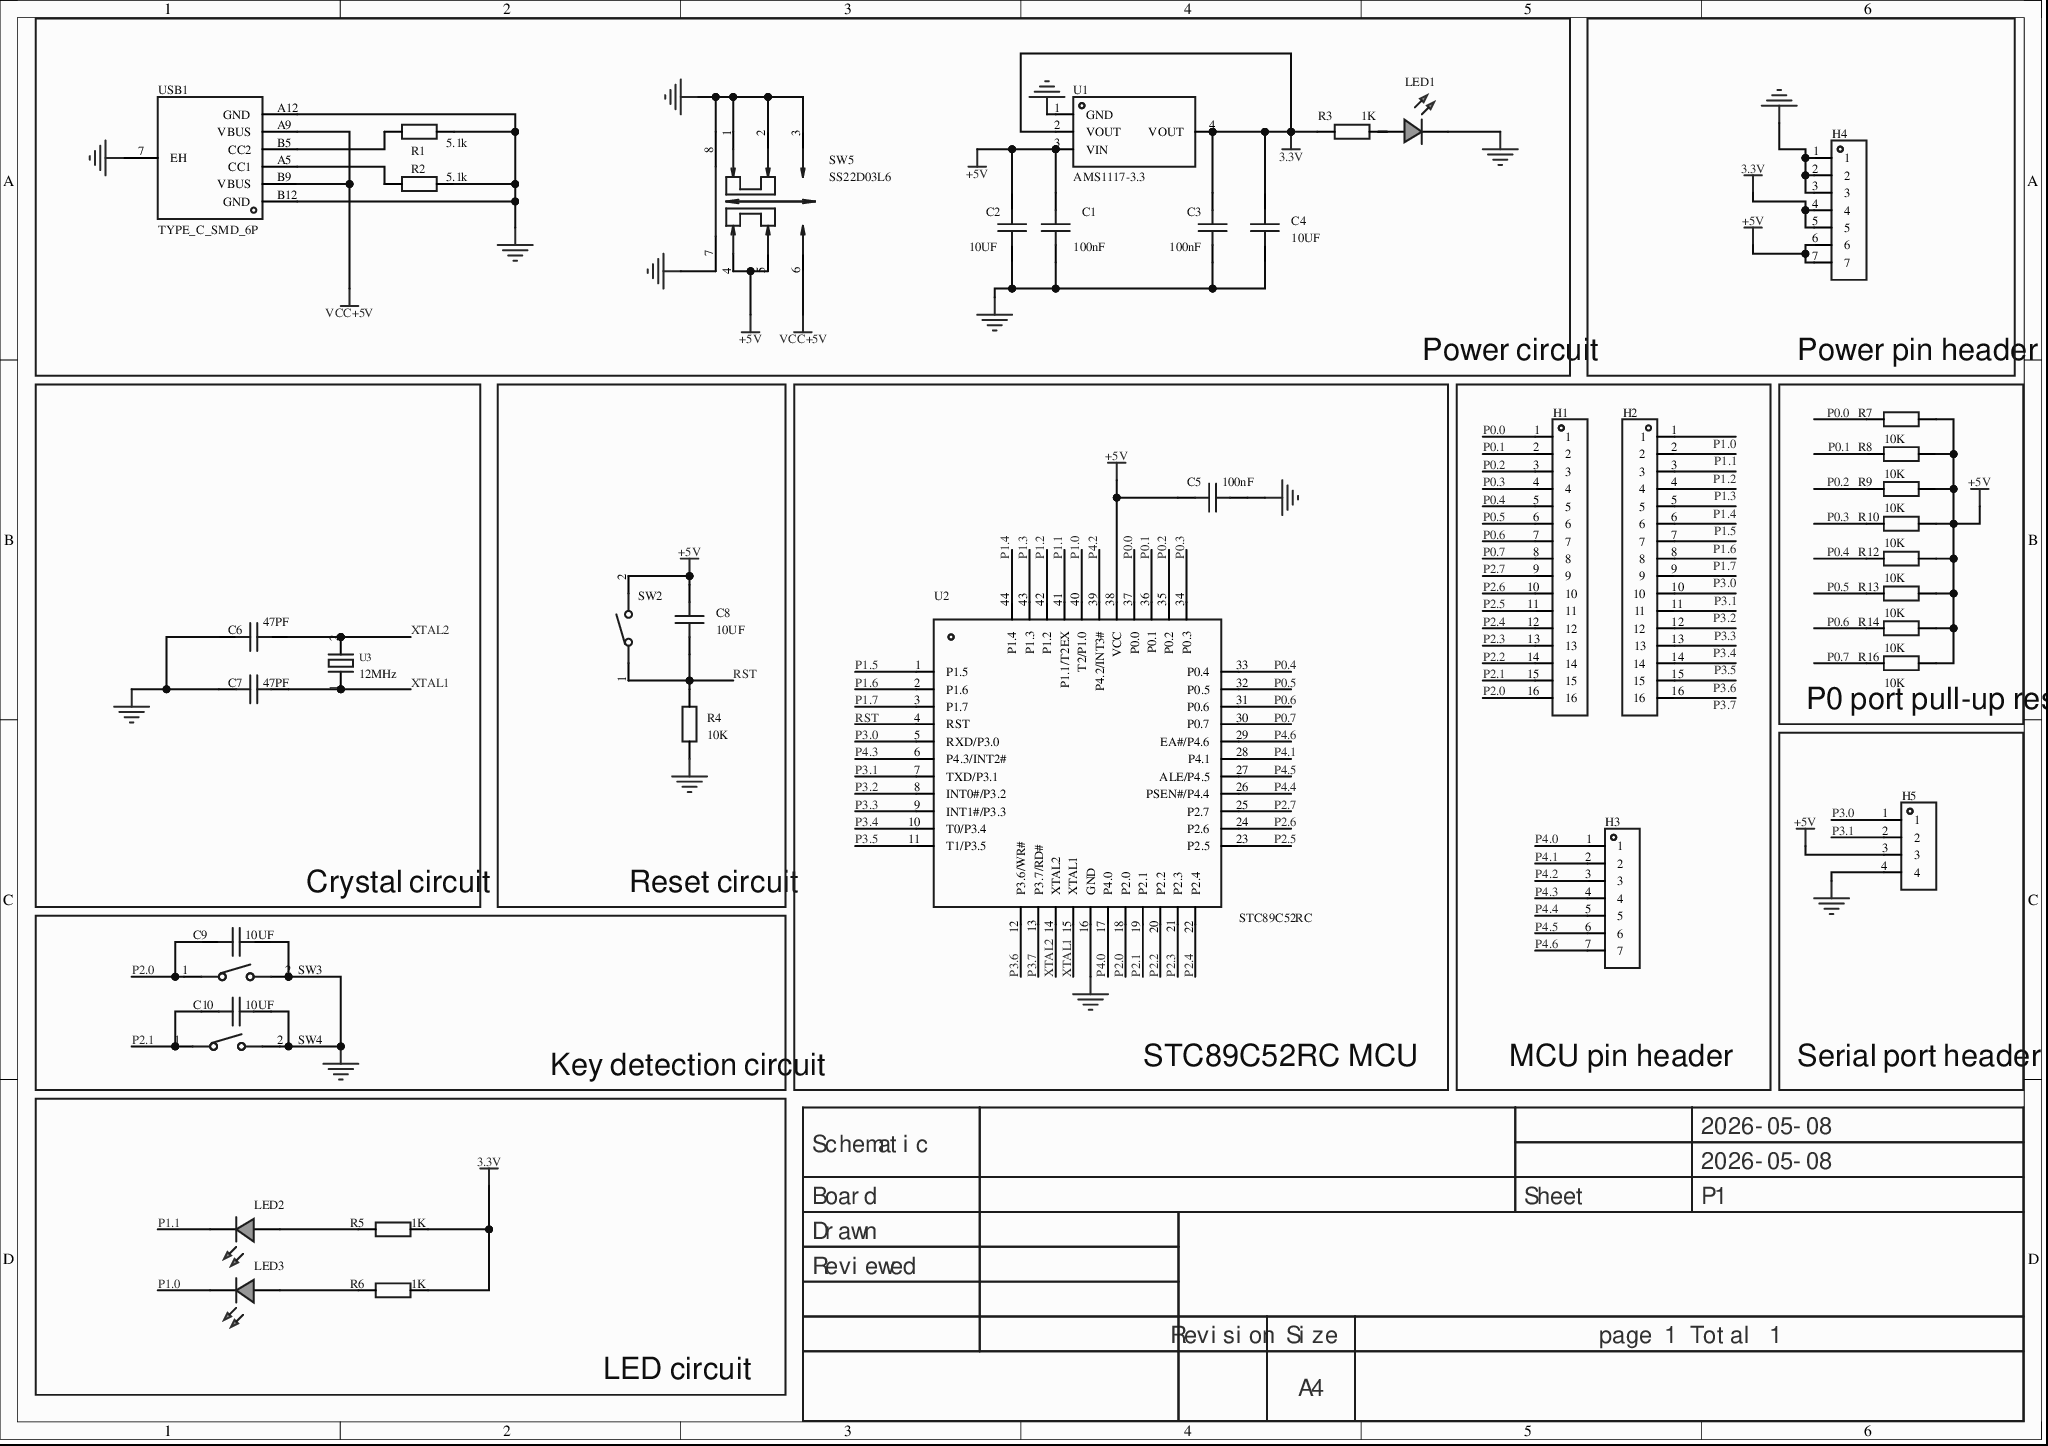
[diagram p0: MISC51716-3.schdoc]
# Altium project MISC51716-2.PrjPcb
1 sheet, 40 parts. Net scope: global (net labels, ports and power ports of the same name join across sheets).
Board file: MISC51716.pcbdoc

## Sheet MISC51716-3.schdoc
size 297 x 209 mm; Version: V1.0; @Project Name: MISC51716; @Update Date: 2026-05-08; @Create Date: 2026-05-08; @Board Name: MISC51716; @Create Time: 11:26:09; @Page Count: 1; @Page No: 1; @Schematic Name: MISC51716; @Update Time: 11:26:09; Size: A4

### Parts
C1  100nF  [C0805]
C2  10UF  [C0805]
C3  100nF  [C0805]
C4  10UF  [C0805]
C5  100nF  [C0805]
C6  47PF  [C0805]
C7  47PF  [C0805]
C8  10UF  [C0805]
C9  10UF  [C0805]
C10  10UF  [C0805]
H1  (no value)  [HDR-TH_16P-P2.54-V-M]
H2  (no value)  [HDR-TH_16P-P2.54-V-M]
H3  (no value)  [HDR-TH_7P-P2.54-V-M]
H4  (no value)  [HDR-TH_7P-P2.54-V-M]
H5  (no value)  [HDR-TH_4P-P2.54-V-M]
LED1  (no value)  [LED_0805]
LED2  (no value)  [LED_0805]
LED3  (no value)  [LED_0805]
R1  5.1k  [R0805]
R2  5.1k  [R0805]
R3  1K  [R0603]
R4  10K  [R0805]
R5  1K  [R0805]
R6  1K  [R0805]
R7  10K  [R0805]
R8  10K  [R0805]
R9  10K  [R0805]
R10  10K  [R0805]
R12  10K  [R0805]
R13  10K  [R0805]
R14  10K  [R0805]
R16  10K  [R0805]
SW2  Tact switch 3*4*H  [SW-SMD_L4.0-W2.9-LS5.0]  (value not drawn)
SW3  Tact switch 3*4*H  [SW-SMD_L4.0-W2.9-LS5.0]  (value not drawn)
SW4  Tact switch 3*4*H  [SW-SMD_L4.0-W2.9-LS5.0]  (value not drawn)
SW5  SS22D03L6  [SW-TH_SS-22D03-L4]
U1  AMS1117-3.3  [SOT-223-3_L6.5-W3.4-P2.30-LS7.0-BR]
U2  STC89C52RC  [LQFP-44_L10.0-W10.0-P0.80-LS12.0-BL]
U3  12MHz  [CRYSTAL-SMD_L11.4-W4.7-LS12.7]
USB1  TYPE_C_SMD_6P  [TYPE-C-SMD_TYPE-C-6P]

### Blocks framed on the sheet
Power circuit: C1-C4 LED1 R1-R3 SW5 U1 USB1
Power pin header: H4
Crystal circuit: C6 C7 U3
Reset circuit: C8 R4 SW2
MCU pin header: H1-H3

### Nets
3.3V: C3.2 C4.2 H4.4 H4.5 R3.1 R5.2 R6.2 U1.2(VOUT) U1.4(VOUT)
+5V: C1.2 C2.2 C5.2 C8.1 H4.6 H4.7 H5.3 R7.1 R8.1 R9.1 R10.1 R12.1 R13.1 R14.1 R16.1 SW2.2 SW5.4 SW5.5 U1.3(VIN) U2.38(VCC)
GND: C1.1 C2.1 C3.1 C4.1 C5.1 C6.2 C7.2 C9.1 C10.1 H4.1 H4.2 H4.3 H5.4 LED1.1(C) R1.2 R2.2 R4.1 SW3.2 SW4.2 SW5.1 SW5.2 SW5.3 SW5.7 SW5.8 U1.1(GND) U2.16(GND) USB1.7(EH) USB1.A12(GND) USB1.B12(GND)
VCC+5V: SW5.6 USB1.A9(VBUS) USB1.B9(VBUS)
P0.0: H1.1 R7.2 U2.37(P0.0)
P0.1: H1.2 R8.2 U2.36(P0.1)
P0.2: H1.3 R9.2 U2.35(P0.2)
P0.3: H1.4 R10.2 U2.34(P0.3)
P0.4: H1.5 R12.2 U2.33(P0.4)
P0.5: H1.6 R13.2 U2.32(P0.5)
P0.6: H1.7 R14.2 U2.31(P0.6)
P0.7: H1.8 R16.2 U2.30(P0.7)
P1.0: H2.1 LED3.1(C) U2.40(T2/P1.0)
P1.1: H2.2 LED2.1(C) U2.41(P1.1/T2EX)
P1.2: H2.3 U2.42(P1.2)
P1.3: H2.4 U2.43(P1.3)
P1.4: H2.5 U2.44(P1.4)
P1.5: H2.6 U2.1(P1.5)
P1.6: H2.7 U2.2(P1.6)
P1.7: H2.8 U2.3(P1.7)
P2.0: C9.2 H1.16 SW3.1 U2.18(P2.0)
P2.1: C10.2 H1.15 SW4.1 U2.19(P2.1)
P2.2: H1.14 U2.20(P2.2)
P2.3: H1.13 U2.21(P2.3)
P2.4: H1.12 U2.22(P2.4)
P2.5: H1.11 U2.23(P2.5)
P2.6: H1.10 U2.24(P2.6)
P2.7: H1.9 U2.25(P2.7)
P3.0: H2.9 H5.1 U2.5(RXD/P3.0)
P3.1: H2.10 H5.2 U2.7(TXD/P3.1)
P3.2: H2.11 U2.8(INT0#/P3.2)
P3.3: H2.12 U2.9(INT1#/P3.3)
P3.4: H2.13 U2.10(T0/P3.4)
P3.5: H2.14 U2.11(T1/P3.5)
P3.6: H2.15 U2.12(P3.6/WR#)
P3.7: H2.16 U2.13(P3.7/RD#)
P4.0: H3.1 U2.17(P4.0)
P4.1: H3.2 U2.28(P4.1)
P4.2: H3.3 U2.39(P4.2/INT3#)
P4.3: H3.4 U2.6(P4.3/INT2#)
P4.4: H3.5 U2.26(PSEN#/P4.4)
P4.5: H3.6 U2.27(ALE/P4.5)
P4.6: H3.7 U2.29(EA#/P4.6)
RST: C8.2 R4.2 SW2.1 U2.4(RST)
XTAL1: C7.1 U2.15(XTAL1) U3.1
XTAL2: C6.1 U2.14(XTAL2) U3.2(GND)
NetLED1_2: LED1.2(A) R3.2
NetLED2_2: LED2.2(A) R5.1
NetLED3_2: LED3.2(A) R6.1
NetR1_1: R1.1 USB1.B5(CC2)
NetR2_1: R2.1 USB1.A5(CC1)

### Notes on the sheet
- (near R16) P0 port pull-up resistors
- Key detection circuit
- STC89C52RC MCU
- Serial port header
- LED circuit
- 2026-05-08
- Schematic
- Board
- Sheet
- P1
- Drawn
- Reviewed
- Revision
- Size
- A4
- page 1 Total 1

### Library data of the parts
C1-C10 = CAP_0805: Symbol: CapAcitance; 3D Model: 1ba041120af144c991958decab20d241; 3D Model Transform: 78.74,51.181,0,0,0,0,0,0.0005,0; ConvertToPcb: yes; ModelName: C0805_L2.0-W1.3-H1.3; Device: CAP_0805; Supplier Footprint: 0805; AddInBom: yes; FootprintName: C0805
  C1 C3 C5: Value: 100nF
  C2 C4 C8-C10: Value: 10UF
  C6 C7: Value: 47PF
H1 H2 = HDR-M_2.54_1x16P: Pitch: 2.54mm; Total pins: 16; Rows: 1; Pin structure: 1x16P; Row spacing: -; Mounting type: Through-hole; Round/square pin: Square; Rated current: 3A; Rated voltage: -; Mating pin length: 6mm; Plastic height: 2.5mm; Termination pin length: 3mm; Contact material: -; Operating temp: -40℃~+105℃; Color: Black;; Symbol: HDR_2.54-1x16P; 3D Model: 8bf9bf52ab1b4a9c8444131cb972ade8; 3D Model Transform: 1590.1543,92.913,0,0,0,0,0,0,-137.795; ConvertToPcb: yes; ModelName: HDR-TH_16P-P2.54-M-LI-1X16P; Device: HDR-M_2.54_1x16P; Supplier Part: C2894939; Supplier Footprint: 插件; AddInBom: yes; FootprintName: HDR-TH_16P-P2.54-V-M
H3 H4 = HDR-M_2.54_1x7P: Symbol: PZ254V-11-07P; 3D Model: 3f496cdc752348c6a5e9157bbaceaf96; 3D Model Transform: 690.1561,98.425,0,0,0,0,0,0,-118.11; ConvertToPcb: yes; ModelName: HDR-TH_7P-P2.54-M-LI-1X7P; Device: HDR-M_2.54_1x7P; Supplier Part: C492406; Supplier Footprint: 插件; AddInBom: yes; FootprintName: HDR-TH_7P-P2.54-V-M
H5 = HDR-M_2.54_1x4P: Symbol: PZ254V-11-04P; 3D Model: 112f4d05e8d64e99ab9a333894bea4f9; 3D Model Transform: 399.999,104.7242,0,0,0,0,0,0,-118.11; ConvertToPcb: yes; ModelName: HDR-TH_4P-P2.54-M-LI-1X4P; Device: HDR-M_2.54_1x4P; Supplier Part: C492403; Supplier Footprint: 插件; AddInBom: yes; FootprintName: HDR-TH_4P-P2.54-V-M
LED1-LED3 = LED_0805-G: Symbol: LED_G; Convert to PCB: yes; 3D Model: 381ae4d721d6485eaad9d0ca067812b5; 3D Model Transform: 63.9,39.8,31.9,0,0,0,0,0,0; ModelName: LED-0805_G; Device: LED_0805-G; Add into BOM: yes; Supplier Footprint: 0805; FootprintName: LED_0805
R1 R2 R4-R10 R12-R14 R16 = Res_0805: Symbol: Resistor; 3D Model: 37a81e68749a4138bd2dfa6897b24b85; 3D Model Transform: 78.74,51.181,0,0,0,0,0,-0.0005,0; ConvertToPcb: yes; ModelName: R0805_L2.0-W1.3-H0.6; Device: Res_0805; Supplier Footprint: 0805; AddInBom: yes; FootprintName: R0805
  R1 R2: Value: 5.1k
  R4 R7-R10 R12-R14 R16: Value: 10K
  R5 R6: Value: 1K
R3 = Res_0603: Symbol: Resistor; 3D Model: fc143cca1e79419f9cd78b61e9279f08; 3D Model Transform: 31.8897,63.7794,0,90,0,0,0,0,0; ConvertToPcb: yes; Device: Res_0603; Value: 1K; Supplier Footprint: 0603; AddInBom: yes; FootprintName: R0603; ModelName: R0603
SW2-SW4 = 轻触按键3*4*H: 3D Model: 63599cce708d48afbce1b0db00354477; 3D Model Transform: 196.85,114.173,0,0,0,0,0,0,0; AddInBom: yes; ModelName: SW-SMD_L4.0-W2.9-H2-LS5.0; Symbol: Tact switch 3*4*H; Device: Tact switch 3*4*H; LCSC Part Name: 轻触按键3*4*H; Supplier Part: C9900017573; Manufacturer Part: 轻触按键3*4*H; Supplier Footprint: 轻触按键3*4*2.5; JLCPCB Part Class: Extended library; Supplier: LCSC; ConvertToPcb: yes; FootprintName: SW-SMD_L4.0-W2.9-LS5.0
SW5 = SS22D03L6: Circuit: DPDT; Mounting: Through-hole; Switch color: Black; Rated current (DC): 300mA; Rated voltage (DC): 50V; Rated current (AC): 300mA; Rated voltage (AC): 50V; Mechanical life: 1万次;; Manufacturer: XKB Connectivity(中国星坤); Symbol: SS-22D03-L6; 3D Model: d0fa754f8b2d49db91271a8678ca589d; 3D Model Transform: 338.582,267.716,0,0,0,0,0,0,-106.299; Actuator Style: Rectangular column; Pin Style: PC pin; Switch Length: 8.6mm; Switch Width: 6.8mm; Switch Height: 4.7mm; AddInBom: yes; Device: SS22D03L6; LCSC Part Name: 柄长6mm 直插双档 滑动开关; Supplier Footprint: 插件; Datasheet: https://example.com/source/20211011/1771D1CCC055340BE9BC64E40A46963B.pdf; Mounting Style: Through-hole; Actuator Color: Black; Current Rating (DC): 300mA; Voltage Rating (DC): 50V; Current Rating (AC): 300mA; Voltage Rating (AC): 50V; Mechanical Life: 1万次; Operating Temperature: -40℃~+85℃; Supplier: LCSC; Supplier Part: C609824; Manufacturer Part: SS22D03L6; JLCPCB Part Class: Extended library; ConvertToPcb: yes; FootprintName: SW-TH_SS-22D03-L4; ModelName: SW-TH_SS-22D03-L4
U1 = AMS1117-3.3_C6186: Output type: Fixed; Max input voltage: -; Output voltage: 3.3V; Max output current: 1A; PSRR: 72dB@(120Hz); Output polarity: Positive;; Manufacturer: AMS; 3D Model: 925194bf9823436183a3e0b978a8d076; 3D Model Transform: 279.89794,255.905,0,180,0,0,-3.9385,-0.0005,0; Dropout Voltage: 1.3V@(800mA); Number of Outputs: 1; AddInBom: yes; ModelName: SOT-223-4P_L6.5-W3.5-H1.6-LS7.0-P2.30; Symbol: AMS1117-3.3; Device: AMS1117-3.3_C6186; LCSC Part Name: 输出3.3V 1A; Supplier Footprint: SOT-223-3; Datasheet: https://example.com/source/20180727/C6186_7A095716F0823C02F1997A905E26C086.pdf; Output Type: Fixed; Maximum Input Voltage: -; Output Voltage: 3.3V; MAX Output Current: 1A; Power Supply Rejection Ratio (PSRR): 72dB@(120Hz); standby current: -; Noise: -; Feature: -; Operating Temperature: -; Output Polarity: Positive; Supplier: LCSC; Manufacturer Part: AMS1117-3.3; Supplier Part: C6186; JLCPCB Part Class: Basic library; ConvertToPcb: yes; FootprintName: SOT-223-3_L6.5-W3.4-P2.30-LS7.0-BR
U2 = STC89C52RC-40I-LQFP44: CPU core: 51 series; Program memory: 8KB; RAM total: 512Byte; GPIO ports: 39; Operating voltage: 3.3V~5.5V; Max CPU frequency: -; Program memory type: FLASH;; Manufacturer: STC(宏晶); Symbol: STC89C52RC-40I_C8707; 3D Model: cfc67ede9fd147078f17820e55193bca; 3D Model Transform: 472.441,472.441,0,0,0,0,0,0,0; GPIO Ports Number: 39; 16Bit Timer: 3; UART/USART: 1; Peripheral/Function: Watchdog; Watchdog: Yes; ModelName: LQFP-44_L10.0-W10.0-H1.4-LS12.0-P0.80; Device: STC89C52RC-40I-LQFP44; Manufacturer Part: STC89C52RC; LCSC Part Name: STC89C52RC-40I-LQFP44; Supplier Part: C8707; Supplier Footprint: LQFP-44(10x10); JLCPCB Part Class: Extended library; Datasheet: https://example.com/source/20131218/1457706663573.pdf; Supplier: LCSC; CPU Core: 51 series; Program Storage Size: 8KB; RAM Size: 512Byte; Operating Voltage Range: 3.3V~5.5V; CPU Maximum Speed: -; Program Memory Type: FLASH; Operating Temperature Range: -40℃~+85℃; ADC (Bit): -; DAC (Bit): -; PWM (Bit): -; 8Bit Timer: -; 32Bit Timer: -; CAN: -; I2C: -; I2S: -; SPI: -; Universal Serial Bus: -; Internal Comparator: -; communication protocol: -; Real-Time Clock: -; Infrared Data Association: -; Low-Voltage Detect: -; CCP Capture/Compare: -; Secure Digital Input and Output: -; Direct Memory Access: -; Internal Oscillator: -; AddInBom: yes; ConvertToPcb: yes; FootprintName: LQFP-44_L10.0-W10.0-P0.80-LS12.0-BL
U3 = ABLS-12.000MHZ-B4H-T: Frequency: 12MHz; Frequency deviation at room temp: ±30ppm; Load capacitance: 18pF; Frequency stability (full temp): ±35ppm;; Manufacturer: ABRACON; 3D Model: be19d32e6d024fb4863eb8f4e3f5efcc; 3D Model Transform: 499.999,185.039,0,0,0,0,0,0,0; Equivalent Series Resistance (ESR): 50Ω; AddInBom: yes; Symbol: ABLS-12.000MHZ-B4H-T; Device: ABLS-12.000MHZ-B4H-T; LCSC Part Name: 12MHz ±30ppm 18pF; Supplier Footprint: HC-49S-SMD; Datasheet: https://example.com/source/20210612/96A8D0E14BE5C26ADD56CBF11909D043.pdf; Normal temperature Frequency Tolerance: ±30ppm; External load capacitor: 18pF; Frequency Stability(Full temperature range): ±35ppm; Operating Temperature: -20℃~+70℃; Supplier: LCSC; Supplier Part: C1986452; Manufacturer Part: ABLS-12.000MHZ-B4H-T; JLCPCB Part Class: Extended library; Value: 12MHz; ConvertToPcb: yes; FootprintName: CRYSTAL-SMD_L11.4-W4.7-LS12.7; ModelName: CRYSTAL-SMD_L11.4-W4.7-LS12.7
USB1 = TYPE_C_SMD_6P: 3D Model: 3770c5585474407db939b2377e27177a; 3D Model Transform: 351.9678,267.716,0,180,0,0,0,-45.766,-39.37; AddInBom: yes; ModelName: TYPE-C-SMD_6P-L8.9-W6.8-H3.2-P1.00; Symbol: TYPE_C_SMD_6P; Device: TYPE_C_SMD_6P; LCSC Part Name: TYPE_C_SMD_6P; Supplier Part: C9900003080; Manufacturer Part: TYPE_C_SMD_6P; Supplier Footprint: TYPE_C_USB_6P; JLCPCB Part Class: Extended library; Supplier: LCSC; ConvertToPcb: yes; FootprintName: TYPE-C-SMD_TYPE-C-6P